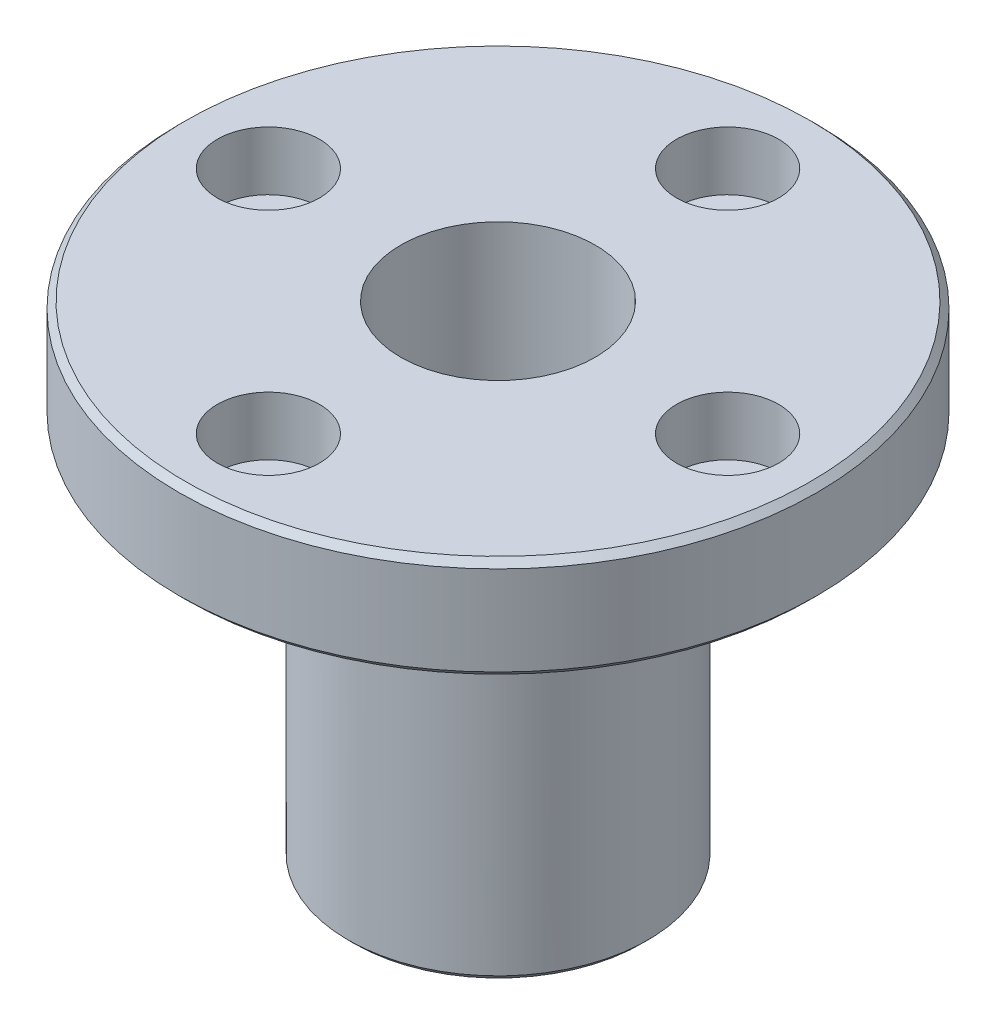
from build123d import *

# Parameters (mm, degrees)
G3_8_TAPPED_HOLE1_D                                 = 15.25
HOLE_SIZE_PER_SOCKET_HEAD_CAP_SCREW_TYP_D           = 4.5
HOLE_SIZE_PER_SOCKET_HEAD_CAP_SCREW_TYP_CBORE_D     = 8
HOLE_SIZE_PER_SOCKET_HEAD_CAP_SCREW_TYP_CBORE_DEPTH = 4.6
CHAMFER1_SIZE                                       = 0.5


with BuildPart() as part:
    # Sketch1 → Revolve1 (revolve)
    with BuildSketch(Plane.XY, mode=Mode.PRIVATE) as revolve1_sk:
        Polygon((0, 38), (-25, 38), (-25, 30), (-11.75, 30), (-11.75, 0), (0, 0), align=None)
    revolve(revolve1_sk.sketch.rotate(Axis((0, 0, 0), (0, 1, 0)), 270), axis=Axis((0, 0, 0), (0, 1, 0)))

    # G3/8 Tapped Hole1 (through all)
    with Locations(Plane.ZX.offset(38)):
        with Locations((0, 0)):
            Hole(G3_8_TAPPED_HOLE1_D / 2)

    # Hole Size (per socket head cap screw type)1 (through all)
    with Locations(Plane(origin=(0, 38, -18), x_dir=(0, 0, 1), z_dir=(0, 1, 0))):
        with Locations((0, 0), (18, -18), (18, 18), (36, 0)):
            CounterBoreHole(HOLE_SIZE_PER_SOCKET_HEAD_CAP_SCREW_TYP_D / 2, HOLE_SIZE_PER_SOCKET_HEAD_CAP_SCREW_TYP_CBORE_D / 2, HOLE_SIZE_PER_SOCKET_HEAD_CAP_SCREW_TYP_CBORE_DEPTH)

    # Chamfer1
    chamfer1_edges = [part.edges().sort_by_distance(p)[0] for p in [
        (0, 0, 11.75),
        (0, 30, 25),
        (0, 38, 25),
    ]]
    chamfer(chamfer1_edges, length=CHAMFER1_SIZE)


solid = part.part
